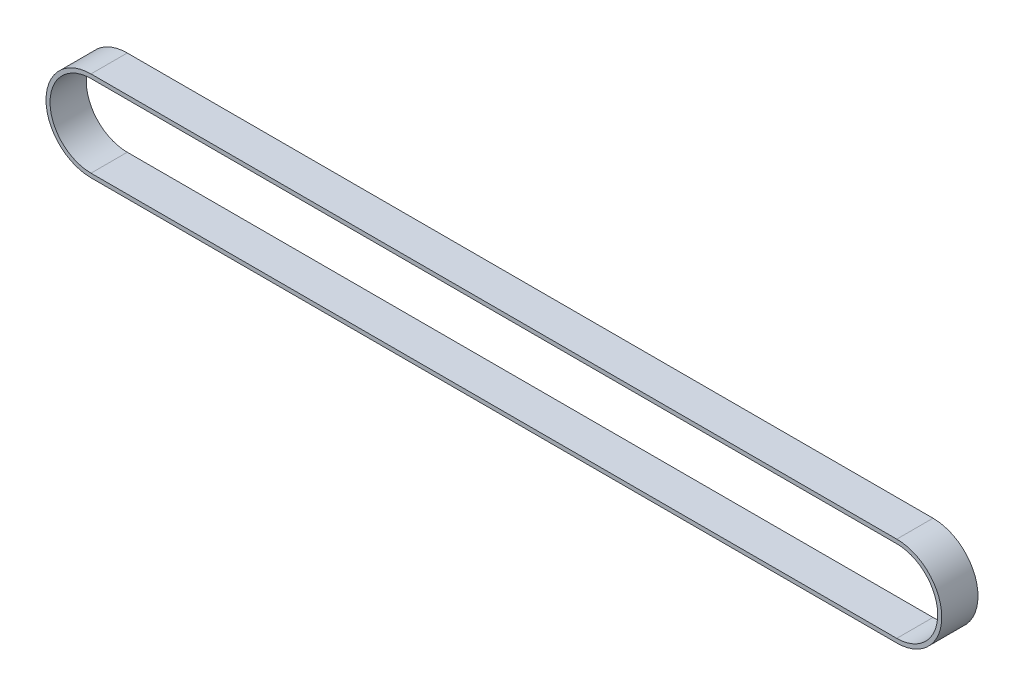
SolidWorks part; units mm, degrees
ref_plane "Front Plane" through (0, 0, 0) normal (0, 0, 1) x (1, 0, 0)
ref_plane "Top Plane" through (0, 0, 0) normal (0, 1, 0) x (1, 0, 0)
ref_plane "Right Plane" through (0, 0, 0) normal (1, 0, 0) x (0, 0, -1)
sketch "Sketch1" plane through (0, 0, 0) normal (0, 0, 1) x (1, 0, 0)
  line L0 (0, 33.5) -> (600, 33.5)
  line L1 (0, -33.5) -> (600, -33.5)
  line L2 (0, 30.5) -> (600, 30.5)
  line L3 (0, -30.5) -> (600, -30.5)
  arc A0 (0, 33.5) -> (0, -33.5) centre (0, 0) ccw
  arc A1 (600, -33.5) -> (600, 33.5) centre (600, 0) ccw
  arc A2 (600, -30.5) -> (600, 30.5) centre (600, 0) ccw
  arc A3 (0, 30.5) -> (0, -30.5) centre (0, 0) ccw
  dimension "D1" = 600
  dimension "D2" = 67
  dimension "D3" = 3
extrude "Boss-Extrude1" add sketch "Sketch1" along normal mid plane 27
